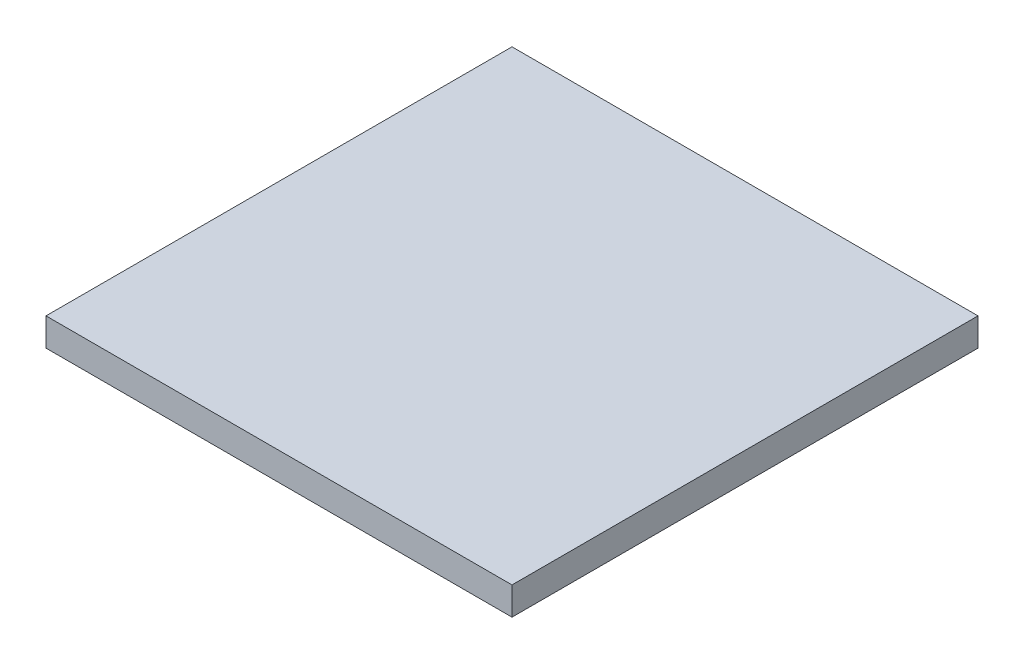
SolidWorks part; units mm, degrees
material "Plain carbon steel"
ref_plane "Front plane" through (0, 0, 0) normal (0, 0, 1) x (1, 0, 0)
ref_plane "Top plane" through (0, 0, 0) normal (0, 1, 0) x (1, 0, 0)
ref_plane "Right plane" through (0, 0, 0) normal (1, 0, 0) x (0, 0, -1)
other "Configuration Table"
sketch "Sketch1" plane through (0, 0, 0) normal (0, 1, 0) x (1, 0, 0)
  line L1 (-25, -25) -> (25, -25)
  line L2 (-25, -25) -> (-25, 25)
  line L3 (-25, 25) -> (25, 25)
  line L4 (25, -25) -> (25, 25)
  line L5 (-25, -25) -> (25, 25) construction
  line L6 (-25, 25) -> (25, -25) construction
  point P0 (0, 0)
  dimension "D1" = 50
  dimension "D2" = 50
extrude "Boss-Extrude1" add sketch "Sketch1" along normal blind 3
